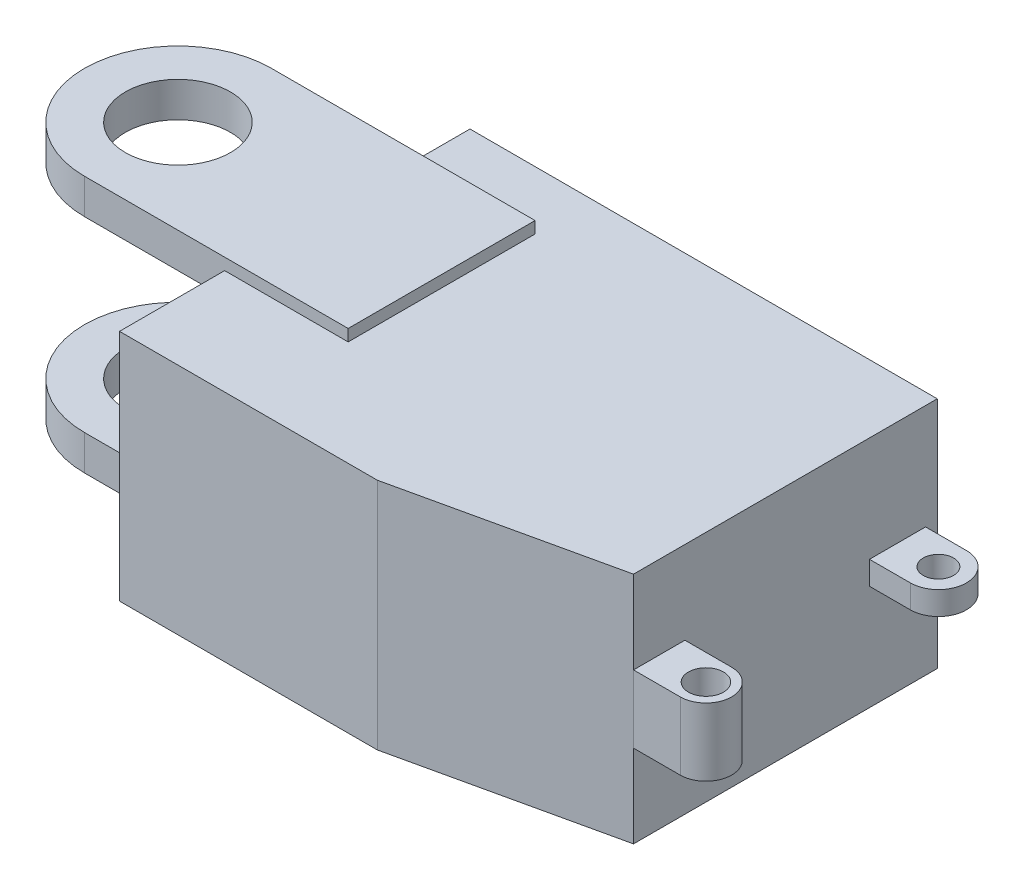
SolidWorks part; units mm, degrees
ref_plane "Front Plane" through (0, 0, 0) normal (0, 0, 1) x (1, 0, 0)
ref_plane "Top Plane" through (0, 0, 0) normal (0, 1, 0) x (1, 0, 0)
ref_plane "Right Plane" through (0, 0, 0) normal (1, 0, 0) x (0, 0, -1)
other "Configuration Table"
sketch "Sketch1" plane through (0, 0, 0) normal (0, 1, 0) x (1, 0, 0)
  line L1 (-200, 150) -> (200, 150)
  line L2 (-200, 150) -> (-200, -150)
  line L3 (-200, -150) -> (200, -150)
  line L4 (200, 150) -> (200, -150)
  line L5 (-200, 150) -> (200, -150) construction
  line L6 (-200, -150) -> (200, 150) construction
  point P0 (0, 0)
  dimension "D1" = 400
  dimension "D2" = 300
extrude "Boss-Extrude1" add sketch "Sketch1" along normal blind 200
ref_plane "Plane1" through (0, 100, 0) normal (0, 1, 0) x (1, 0, 0)
sketch "Sketch2" plane through (0, 100, 0) normal (0, 1, 0) x (1, 0, 0)
  line L0 (134.7229, -88) -> (240, -88) construction
  line L1 (187.3614, -66) -> (240, -66)
  line L2 (187.3614, -110) -> (240, -110)
  line L3 (-200, -150) -> (200, -150) construction
  line L4 (200, -150) -> (200, 150) construction
  line L5 (187.3614, -66) -> (187.3614, -110)
  arc A1 (240, -110) -> (240, -66) centre (240, -88) ccw
  circle A2 centre (240, -88) radius 15
  point P2 (187.3614, -88)
  dimension "D2" = 22
  dimension "D4" = 30
  dimension "D1" = 40
  dimension "D3" = 40
extrude "Boss-Extrude2" add sketch "Sketch2" along normal blind 29 and the other way blind 29
sketch "Sketch3" plane through (0, 200, 0) normal (0, 1, 0) x (1, 0, 0)
  line L0 (200, -110) -> (20.7287, -150)
  line L1 (-200, -150) -> (200, -150) construction
  line L2 (20.7287, -150) -> (200, -150)
  line L3 (200, -150) -> (200, -110)
extrude "Cut-Extrude1" cut sketch "Sketch3" against normal through all
sketch "Sketch4" plane through (0, 200, 0) normal (0, 1, 0) x (1, 0, 0)
  line L0 (-200, 20) -> (200, 20) construction
  line L3 (-200, 150) -> (-200, -150) construction
  line L4 (200, -110) -> (200, 150) construction
  line L5 (-94.2786, 20) -> (-320, 20) construction
  line L6 (-94.2786, -60) -> (-320, -60)
  line L7 (-94.2786, 100) -> (-320, 100)
  line L8 (-94.2786, 100) -> (-94.2786, -60)
  arc A1 (-320, 100) -> (-320, -60) centre (-320, 20) ccw
  circle A2 centre (-320, 20) radius 45
  point P8 (-207.1393, 20)
  dimension "D1" = 80
  dimension "D2" = 120
extrude "Boss-Extrude3" add sketch "Sketch4" against normal blind 20 and the other way blind 10
mirror "Mirror1" about plane through (0, 100, 0) normal (0, 1, 0) of "Boss-Extrude3"
sketch "Sketch5" plane through (0, 100, 0) normal (0, 1, 0) x (1, 0, 0)
  line L0 (133.4956, 116) -> (235, 116) construction
  line L1 (184.2478, 140) -> (235, 140)
  line L2 (184.2478, 92) -> (235, 92)
  line L3 (200, 150) -> (-200, 150) construction
  line L4 (200, -110) -> (200, 150) construction
  line L5 (184.2478, 140) -> (184.2478, 92)
  arc A1 (235, 92) -> (235, 140) centre (235, 116) ccw
  circle A2 centre (235, 116) radius 13
  point P2 (184.2478, 116)
  dimension "D1" = 24
  dimension "D2" = 26
  dimension "D3" = 10
  dimension "D4" = 35
extrude "Boss-Extrude4" add sketch "Sketch5" along normal blind 10 and the other way blind 10
